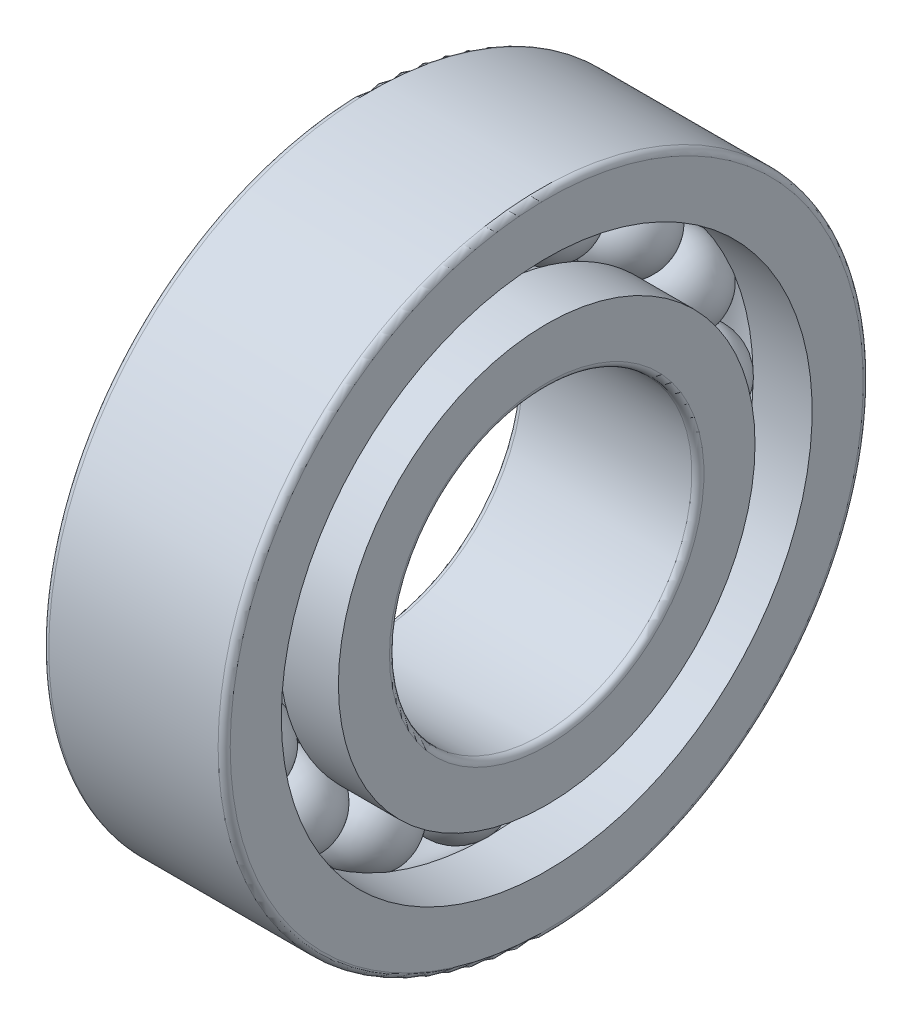
from build123d import *

# Parameters (mm, degrees)
CIRCULAR_PATTERN1_COUNT = 16
FILLET1_R               = 0.3


with BuildPart() as part:
    # Sketch1 → Revolve1 (revolve)
    with BuildSketch(Plane.XY):
        with BuildLine():
            Line((-2.125, 11.749999999999996), (2.125, 11.749999999999996))
            ThreePointArc((2.125, 11.749999999999996), (1.3e-16, 13.874999999999996), (-2.125, 11.749999999999996))
        make_face()
    revolve1 = revolve(axis=Axis((-4.596601835273904, 11.749999999999996, 0), (1, 0, 0)))

    # Sketch2 → Revolve2 (revolve)
    with BuildSketch(Plane.XY, mode=Mode.PRIVATE) as revolve2_sk:
        with BuildLine():
            Line((-4.500000000000001, 10.333333333333334), (-4.500000000000001, 7.5))
            Line((-4.500000000000001, 7.5), (4.499999999999996, 7.5))
            Line((4.499999999999996, 7.5), (4.499999999999997, 10.333333333333334))
            Line((4.499999999999997, 10.333333333333334), (1.5704396058287506, 10.333333333333334))
            ThreePointArc((1.5704396058287506, 10.333333333333334), (1.3e-16, 9.634999999999998), (-1.5704396058287506, 10.333333333333334))
            Line((-1.5704396058287506, 10.333333333333334), (-4.500000000000001, 10.333333333333334))
        make_face()
    revolve(revolve2_sk.sketch.rotate(Axis((-6.971390126215839, 0, 0), (1, 0, 0)), 90), axis=Axis((-6.971390126215839, 0, 0), (1, 0, 0)))

    # Sketch3 → Revolve3 (revolve)
    with BuildSketch(Plane.XY, mode=Mode.PRIVATE) as revolve3_sk:
        with BuildLine():
            Line((-4.500000000000002, 16), (4.499999999999997, 16))
            Line((4.499999999999997, 16), (4.499999999999999, 13.16666666666666))
            Line((4.499999999999999, 13.16666666666666), (1.570439605828751, 13.16666666666666))
            ThreePointArc((1.570439605828751, 13.16666666666666), (1.3e-16, 13.864999999999997), (-1.570439605828751, 13.16666666666666))
            Line((-1.570439605828751, 13.16666666666666), (-4.500000000000001, 13.16666666666666))
            Line((-4.500000000000001, 13.16666666666666), (-4.500000000000002, 16))
        make_face()
    revolve(revolve3_sk.sketch.rotate(Axis((-8.710676494715049, 0, 0), (1, 0, 0)), 90), axis=Axis((-8.710676494715049, 0, 0), (1, 0, 0)))

    # Circular-Pattern1: Revolve1 ×16 about axis
    circular_pattern1_axis = Axis((0, -1.1e-16, 9e-17), (1, 0, 0))
    for i in range(1, CIRCULAR_PATTERN1_COUNT):
        add(revolve1.rotate(circular_pattern1_axis, i * 360 / CIRCULAR_PATTERN1_COUNT))

    # Fillet1
    fillet1_edges = [part.edges().sort_by_distance(p)[0] for p in [
        (-4.500000000000002, -3.74e-15, -16),
        (4.4999999999999964, -3.74e-15, -16),
        (-4.500000000000001, -5.08e-15, -7.5),
        (4.499999999999995, -5.08e-15, -7.5),
    ]]
    fillet(fillet1_edges, radius=FILLET1_R)


solid = part.part
